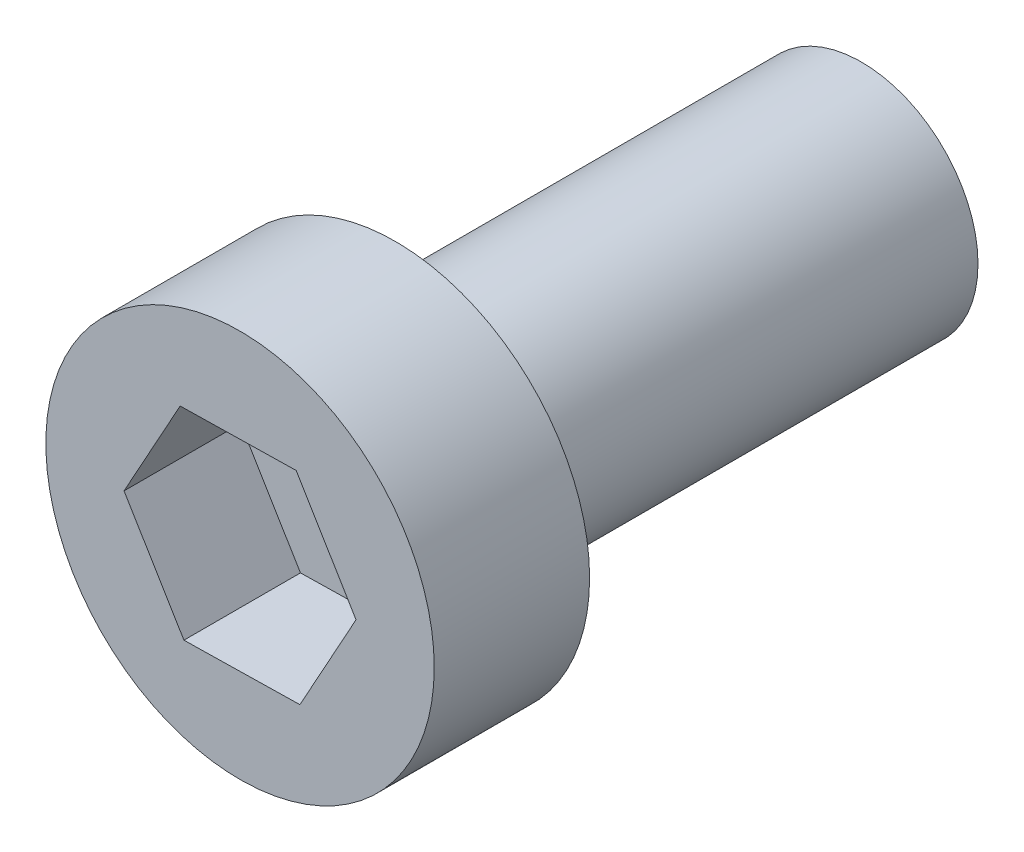
SolidWorks part; units mm, degrees
ref_plane "Front Plane" through (0, 0, 0) normal (0, 0, 1) x (1, 0, 0)
ref_plane "Top Plane" through (0, 0, 0) normal (0, 1, 0) x (1, 0, 0)
ref_plane "Right Plane" through (0, 0, 0) normal (1, 0, 0) x (0, 0, -1)
other "Configuration Table"
sketch "Sketch1" plane through (0, 0, 0) normal (0, 0, 1) x (1, 0, 0)
  circle A0 centre (0, 0) radius 1.5
extrude "Boss-Extrude1" add sketch "Sketch1" against normal blind 6
sketch "Sketch2" plane through (0, 0, 0) normal (0, 0, 1) x (1, 0, 0)
  circle A0 centre (0, 0) radius 2.5
extrude "Boss-Extrude2" add sketch "Sketch2" along normal blind 2
sketch "Sketch3" plane through (0, 0, 2) normal (0, 0, 1) x (1, 0, 0)
  line L1 (0.7223, 1.3072) -> (-0.7709, 1.2791)
  line L2 (-0.7709, 1.2791) -> (-1.4932, -0.0281)
  line L3 (-1.4932, -0.0281) -> (-0.7223, -1.3072)
  line L4 (-0.7223, -1.3072) -> (0.7709, -1.2791)
  line L5 (0.7709, -1.2791) -> (1.4932, 0.0281)
  line L6 (1.4932, 0.0281) -> (0.7223, 1.3072)
  circle A0 centre (0, 0) radius 1.2934 construction
extrude "Cut-Extrude1" cut sketch "Sketch3" against normal blind 1.5
